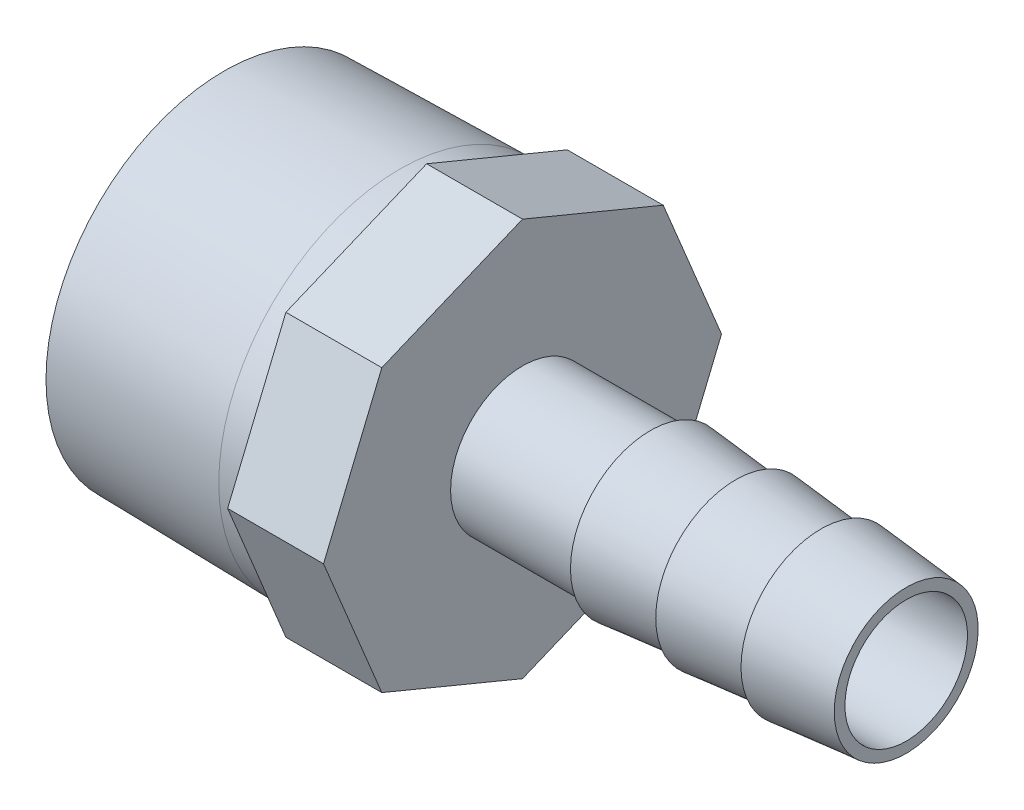
SolidWorks part; units mm, degrees
material "PP 共聚物"
ref_plane "Front Plane" through (0, 0, 0) normal (0, 0, 1) x (1, 0, 0)
ref_plane "Top Plane" through (0, 0, 0) normal (0, 1, 0) x (1, 0, 0)
ref_plane "Right Plane" through (0, 0, 0) normal (1, 0, 0) x (0, 0, -1)
sketch "Sketch1" plane through (0, 0, 0) normal (0, 0, 1) x (1, 0, 0)
  line L0 (19, 17) -> (19, 17.25)
  line L1 (19, 17.25) -> (28, 17.25)
  line L2 (28, 17.25) -> (28, 6.75)
  line L3 (56, 7.5) -> (-16.368, 7.5) construction
  line L4 (56, 7.5) -> (56, 6.75)
  line L5 (56, 7.5) -> (64, 6.75)
  line L6 (16.5, 17) -> (0, 16.712)
  line L7 (0, 16.712) -> (0, 14)
  line L8 (64, 6.75) -> (64, 5.75)
  line L9 (64, 5.75) -> (26, 5.75)
  line L10 (0, 0) -> (121.5719, 0) construction
  line L11 (19, 17) -> (16.5, 17)
  line L12 (26, 5.75) -> (26, 14)
  line L13 (56, 6.75) -> (48, 7.5)
  line L14 (48, 7.5) -> (48, 6.75)
  line L15 (40, 6.75) -> (28, 6.75)
  line L16 (48, 6.75) -> (40, 7.5)
  line L17 (40, 7.5) -> (40, 6.75)
  line L18 (26, 14) -> (0, 14)
  line L19 (0, 14) -> (0, 0) construction
  dimension "D4" = 2.5
  dimension "D9" = 19
  dimension "D1" = 9
  dimension "D2" = 34
  dimension "D3" = 34.5
  dimension "D5" = 15
  dimension "D6" = 36
  dimension "D7" = 13.5
  dimension "D8" = 8
  dimension "D10" = 89
  dimension "D11" = 28
  dimension "D12" = 2
  dimension "D13" = 11.5
revolve "Revolve1" add sketch "Sketch1" angle 360 about L10
ref_plane "Plane1" through (23.5, 0, 0) normal (-1, 0, 0) x (0, 0, 1)
sketch "Sketch4" plane through (28, 0, 0) normal (1, 0, 0) x (0, 0, -1)
  line L1 (0, 18.6713) -> (-13.2026, 13.2026)
  line L2 (-13.2026, 13.2026) -> (-18.6713, 0)
  line L3 (-18.6713, 0) -> (-13.2026, -13.2026)
  line L4 (-13.2026, -13.2026) -> (0, -18.6713)
  line L5 (0, -18.6713) -> (13.2026, -13.2026)
  line L6 (13.2026, -13.2026) -> (18.6713, 0)
  line L7 (18.6713, 0) -> (13.2026, 13.2026)
  line L8 (13.2026, 13.2026) -> (0, 18.6713)
  circle A0 centre (0, 0) radius 17.25 construction
  circle A1 centre (0, 0) radius 17.25 construction
  circle A4 centre (0, 0) radius 17 construction
  circle A5 centre (0, 0) radius 17
extrude "Boss-Extrude1" add sketch "Sketch4" against normal up to surface (9 mm away) up to face at (19, 0, 17)
